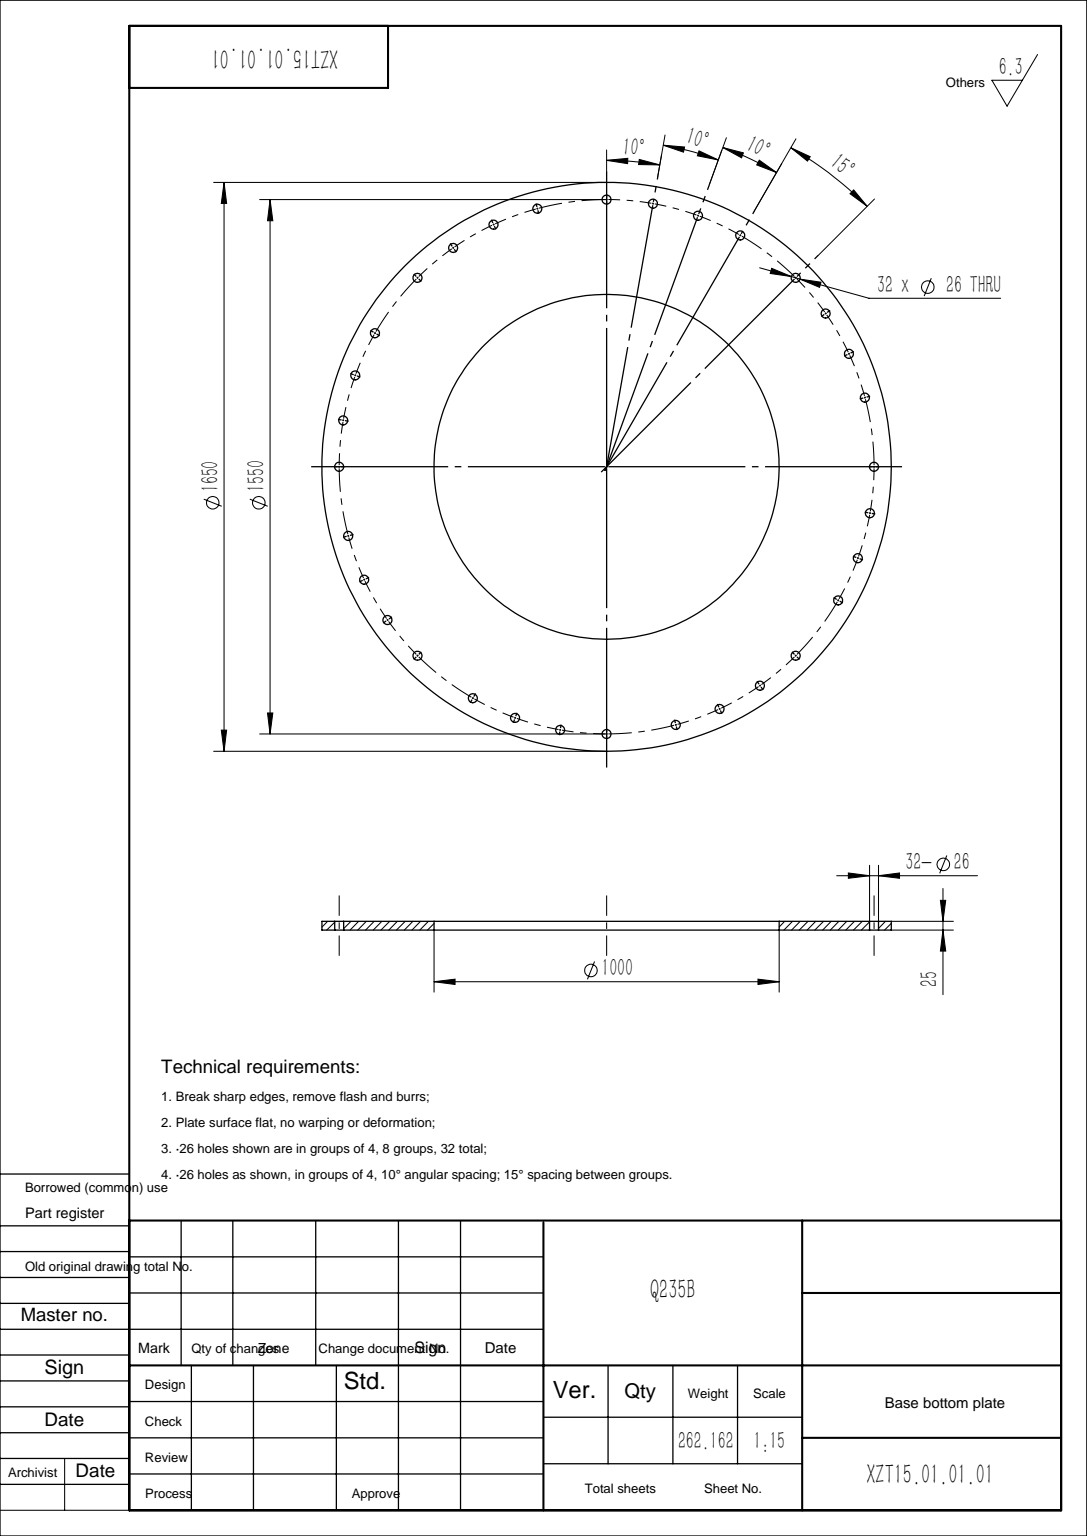
SolidWorks part; units mm, degrees
material "Q235B"
ref_plane "Front Plane" through (0, 0, 0) normal (0, 0, 1) x (1, 0, 0)
ref_plane "Top Plane" through (0, 0, 0) normal (0, 1, 0) x (1, 0, 0)
ref_plane "Right Plane" through (0, 0, 0) normal (1, 0, 0) x (0, 0, -1)
sketch "Sketch1" plane through (0, 0, 0) normal (0, 1, 0) x (1, 0, 0)
  circle A0 centre (0, 0) radius 825
  circle A1 centre (0, 0) radius 500
  dimension "D1" = 1650
  dimension "D2" = 1000
extrude "Boss-Extrude1" add sketch "Sketch1" along normal blind 25
hole_wizard "Ø24.5 (24.5) Diameter Hole1" positions "Sketch2" profile "Sketch3" hole size "Ø24.5" standard "GB" end condition up to next
sketch "Sketch2" plane through (0, 25, 0) normal (0, 1, 0) x (1, 0, 0)
  line L0 (0, 0) -> (0, 775) construction
  line L1 (0, 0) -> (134.5773, 763.226) construction
  circle A1 centre (0, 0) radius 775 construction
  point P0 (0, 775)
  point P13 (134.5773, 763.226)
  point P14 (265.0656, 728.2618)
  point P15 (387.5, 671.1697)
  point P26 (548.0078, 548.0078)
  point P27 (634.8428, 444.5217)
  point P28 (702.3885, 327.5292)
  point P29 (748.5925, 200.5848)
  point P30 (775, 0)
  point P31 (763.226, -134.5773)
  point P32 (728.2618, -265.0656)
  point P33 (671.1697, -387.5)
  point P34 (548.0078, -548.0078)
  point P35 (444.5217, -634.8428)
  point P36 (327.5292, -702.3885)
  point P37 (200.5848, -748.5925)
  point P38 (0, -775)
  point P39 (-134.5773, -763.226)
  point P40 (-265.0656, -728.2618)
  point P41 (-387.5, -671.1697)
  point P42 (-548.0078, -548.0078)
  point P43 (-634.8428, -444.5217)
  point P44 (-702.3885, -327.5292)
  point P45 (-748.5925, -200.5848)
  point P46 (-775, 0)
  point P47 (-763.226, 134.5773)
  point P48 (-728.2618, 265.0656)
  point P49 (-671.1697, 387.5)
  point P50 (-548.0078, 548.0078)
  point P51 (-444.5217, 634.8428)
  point P52 (-327.5292, 702.3885)
  point P53 (-200.5848, 748.5925)
  dimension "D1" = 1550
  dimension "D3" = 10
  dimension "D2" = 4
  dimension "D4" = 8
sketch "Sketch3" plane through (0, 25, -775) normal (1, 0, 0) x (0, 0, 1)
  line L0 (0, 0) -> (0, 25)
  line L1 (0, 25) -> (13, 25)
  line L2 (13, 25) -> (13, 0)
  line L5 (13, 0) -> (0, 0)
  line L11 (0, -6.35) -> (0, 107.95) construction
  dimension "通孔孔直径" = 26
  dimension "通孔孔深度" = 25
